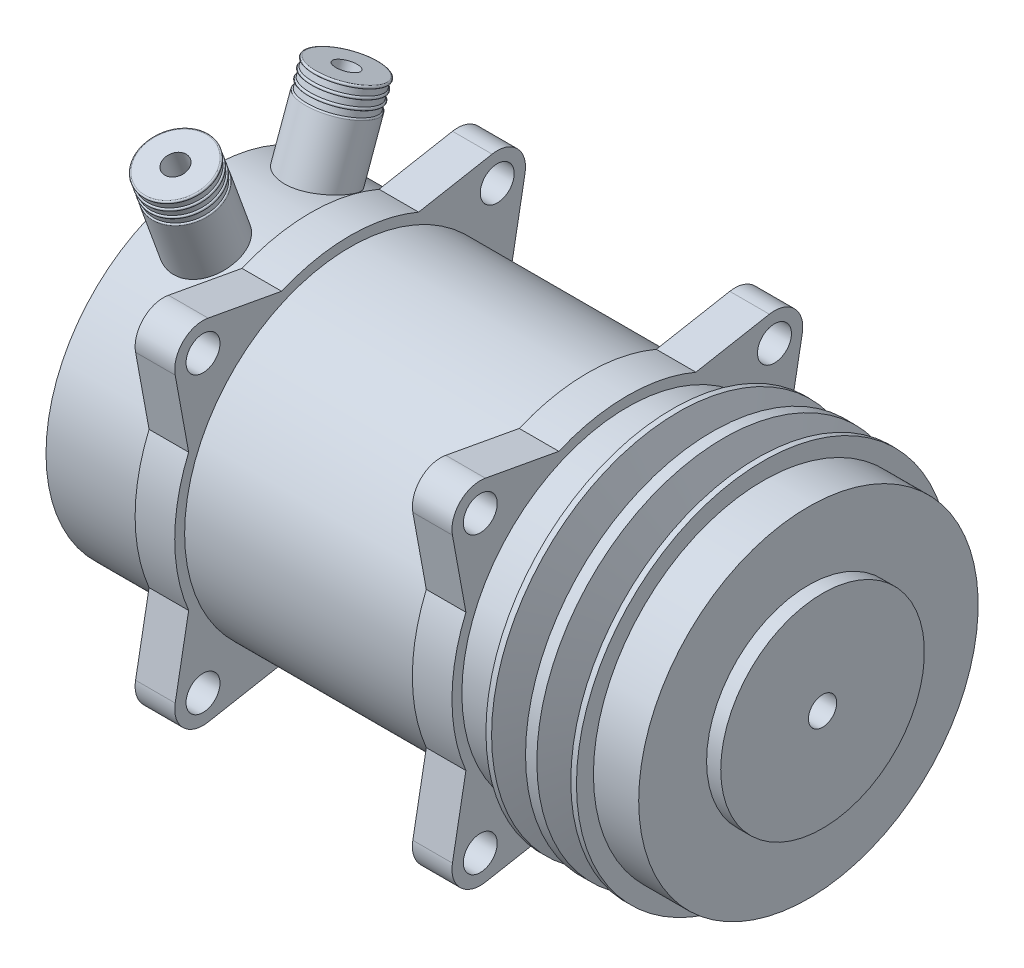
SolidWorks part; units mm, degrees
material "45"
ref_plane "Front Plane" through (0, 0, 0) normal (0, 0, 1) x (1, 0, 0)
ref_plane "Top Plane" through (0, 0, 0) normal (0, 1, 0) x (1, 0, 0)
ref_plane "Right Plane" through (0, 0, 0) normal (1, 0, 0) x (0, 0, -1)
sketch "Sketch1" plane through (0, 0, 0) normal (1, 0, 0) x (0, 0, -1)
  circle A0 centre (0, 0) radius 58.5
  dimension "D1" = 117
extrude "Boss-Extrude1" add sketch "Sketch1" against normal blind 147
sketch "Sketch2" plane through (0, 0, 0) normal (1, 0, 0) x (0, 0, -1)
  circle A0 centre (0, 0) radius 58.5 construction
  circle A1 centre (0, 0) radius 58.5
extrude "Boss-Extrude2" add sketch "Sketch2" along normal blind 16
sketch "Sketch3" plane through (0, 0, 0) normal (0, 0, 1) x (1, 0, 0)
  line L0 (-162.7805, 0) -> (95.2808, 0) construction
  line L1 (50, 0) -> (-50, 0) construction
  line L2 (16, 58.5) -> (-147, 58.5) construction
  line L5 (16, 58.5) -> (-147, 58.5) construction
  line L6 (0, 86.7846) -> (0, -86.1126) construction
  line L7 (0, -50) -> (0, 50) construction
  line L8 (16, 5) -> (16, 66)
  line L9 (0, 62) -> (-14, 62)
  line L10 (0, 62) -> (0, 58.5)
  line L11 (0, 58.5) -> (-14, 58.5)
  line L12 (-14, 62) -> (-14, 58.5)
  line L13 (-98, 58.5) -> (-112, 58.5)
  line L14 (-98, 58.5) -> (-98, 62)
  line L15 (-98, 62) -> (-112, 62)
  line L16 (-112, 58.5) -> (-112, 62)
  line L17 (16, 66) -> (18, 66)
  line L18 (18, 66) -> (21.899, 54)
  line L19 (21.899, 54) -> (26.101, 54)
  line L20 (26.101, 54) -> (30, 66)
  line L21 (30, 66) -> (34, 66)
  line L22 (34, 66) -> (37.899, 54)
  line L23 (37.899, 54) -> (42.101, 54)
  line L24 (42.101, 54) -> (46, 66)
  line L25 (46, 66) -> (48, 66)
  line L26 (48, 66) -> (48, 60)
  line L27 (48, 60) -> (64, 60)
  line L28 (64, 60) -> (64, 36)
  line L29 (64, 36) -> (69, 36)
  line L30 (69, 36) -> (69, 5)
  line L31 (16, 5) -> (69, 5)
  dimension "D2" = 14
  dimension "D3" = 124
  dimension "D4" = 112
  dimension "D5" = 72
  dimension "D6" = 120
  dimension "D7" = 132
  dimension "D8" = 14
  dimension "D9" = 4
  dimension "D10" = 2
  dimension "D11" = 14
  dimension "D12" = 108
  dimension "D13" = 36
  dimension "D14" = 48
  dimension "D15" = 69
  dimension "D16" = 36
  dimension "D17" = 10
  dimension "D18" = 14
revolve "Revolve1" add sketch "Sketch3" angle 360 about L0
ref_plane "Plane1" through (-129.5, 0, 0) normal (1, 0, 0) x (0, 0, -1)
sketch "Sketch5" plane through (-129.5, 0, 0) normal (1, 0, 0) x (0, 0, -1)
  line L2 (-31.7978, 87.3636) -> (0, 0) construction
  line L3 (0, 88.6712) -> (0, -74.8018) construction
  line L4 (0, 50) -> (0, -50) construction
  line L6 (-18.9583, 87.1731) -> (-41.5109, 78.9646) construction
  line L7 (-18.9583, 87.1731) -> (-5.2775, 49.5854) construction
  line L8 (-41.5109, 78.9646) -> (-27.8301, 41.3769) construction
  line L9 (-5.2775, 49.5854) -> (-27.8301, 41.3769) construction
  line L10 (-40.87, 78.6657) -> (-27.5313, 42.0177) construction
  line L11 (-5.9183, 49.8842) -> (-27.5313, 42.0177) construction
  line L12 (-19.2571, 86.5322) -> (-5.9183, 49.8842) construction
  line L13 (-19.2571, 86.5322) -> (-40.87, 78.6657) construction
  line L14 (-18.231, 83.7131) -> (-39.844, 75.8467) construction
  line L15 (-17.205, 80.8941) -> (-38.8179, 73.0276) construction
  line L16 (-16.1789, 78.075) -> (-37.7919, 70.2085) construction
  line L17 (-33.9934, 81.7007) -> (-41.041, 79.1356)
  line L18 (-40.699, 78.1959) -> (-40.015, 76.3165)
  line L19 (-39.673, 75.3768) -> (-38.9889, 73.4974)
  line L20 (-38.6469, 72.5577) -> (-37.9629, 70.6784)
  line L21 (-38.2617, 70.0375) -> (-27.8301, 41.3769)
  line L22 (-27.8301, 41.3769) -> (-20.3125, 44.113)
  line L23 (-33.9934, 81.7007) -> (-20.3125, 44.113)
  arc A0 (-41.041, 79.1356) -> (-40.699, 78.1959) centre (-40.87, 78.6657) ccw
  arc A1 (-40.015, 76.3165) -> (-39.673, 75.3768) centre (-39.844, 75.8467) ccw
  arc A2 (-38.9889, 73.4974) -> (-38.6469, 72.5577) centre (-38.8179, 73.0276) ccw
  arc A3 (-37.9629, 70.6784) -> (-38.2617, 70.0375) centre (-37.7919, 70.2085) ccw
  dimension "D1" = 20
  dimension "D2" = 88.4
  dimension "D3" = 24
  dimension "D4" = 40
  dimension "D8" = 3
  dimension "D9" = 4
  dimension "D5" = 0.5
  dimension "D6" = 3
  dimension "D7" = 3
revolve "Revolve2" add sketch "Sketch5" angle 360 about L2
mirror "Mirror1" about plane through (0, 0, 0) normal (0, 0, 1) of "Revolve2"
sketch "Sketch6" plane through (0, 0, 0) normal (1, 0, 0) x (0, 0, -1)
  line L0 (-56.3893, 20.5) -> (-49.7644, 13.8752)
  line L1 (-110.0209, 0) -> (102.6375, 0) construction
  line L2 (-49.7644, 13.8752) -> (-13.8752, 49.7644)
  line L3 (0, 99.4291) -> (0, -92.5962) construction
  line L4 (0, 50) -> (0, -50) construction
  line L5 (-13.8752, 49.7644) -> (-20.5, 56.3893)
  line L6 (-56.3893, 20.5) -> (-61.8359, 50.196)
  line L7 (-20.5, 56.3893) -> (-50.196, 61.8359)
  circle A0 centre (0, 0) radius 60 construction
  arc A1 (-20.5, 56.3893) -> (-56.3893, 20.5) centre (0, 0) ccw construction
  circle A3 centre (-52, 52) radius 6
  arc A7 (-50.196, 61.8359) -> (-61.8359, 50.196) centre (-52, 52) ccw
  circle A9 centre (0, 0) radius 60 construction
  dimension "D1" = 45
  dimension "D3" = 12
  dimension "D6" = 41
  dimension "D8" = 10
  dimension "D2" = 45
  dimension "D4" = 104
  dimension "D5" = 104
  dimension "D7" = 41
extrude "Boss-Extrude3" add sketch "Sketch6" against normal blind 14
mirror "Mirror2" about plane through (0, 0, 0) normal (0, 0, 1) of "Boss-Extrude3"
mirror "Mirror3" about plane through (0, 0, 0) normal (0, 1, 0) of "Mirror2", "Boss-Extrude3"
pattern_linear "LPattern1" count 2 spacing 98 along (-1, 0, 0) of "Mirror3", "Boss-Extrude3", "Mirror2"
